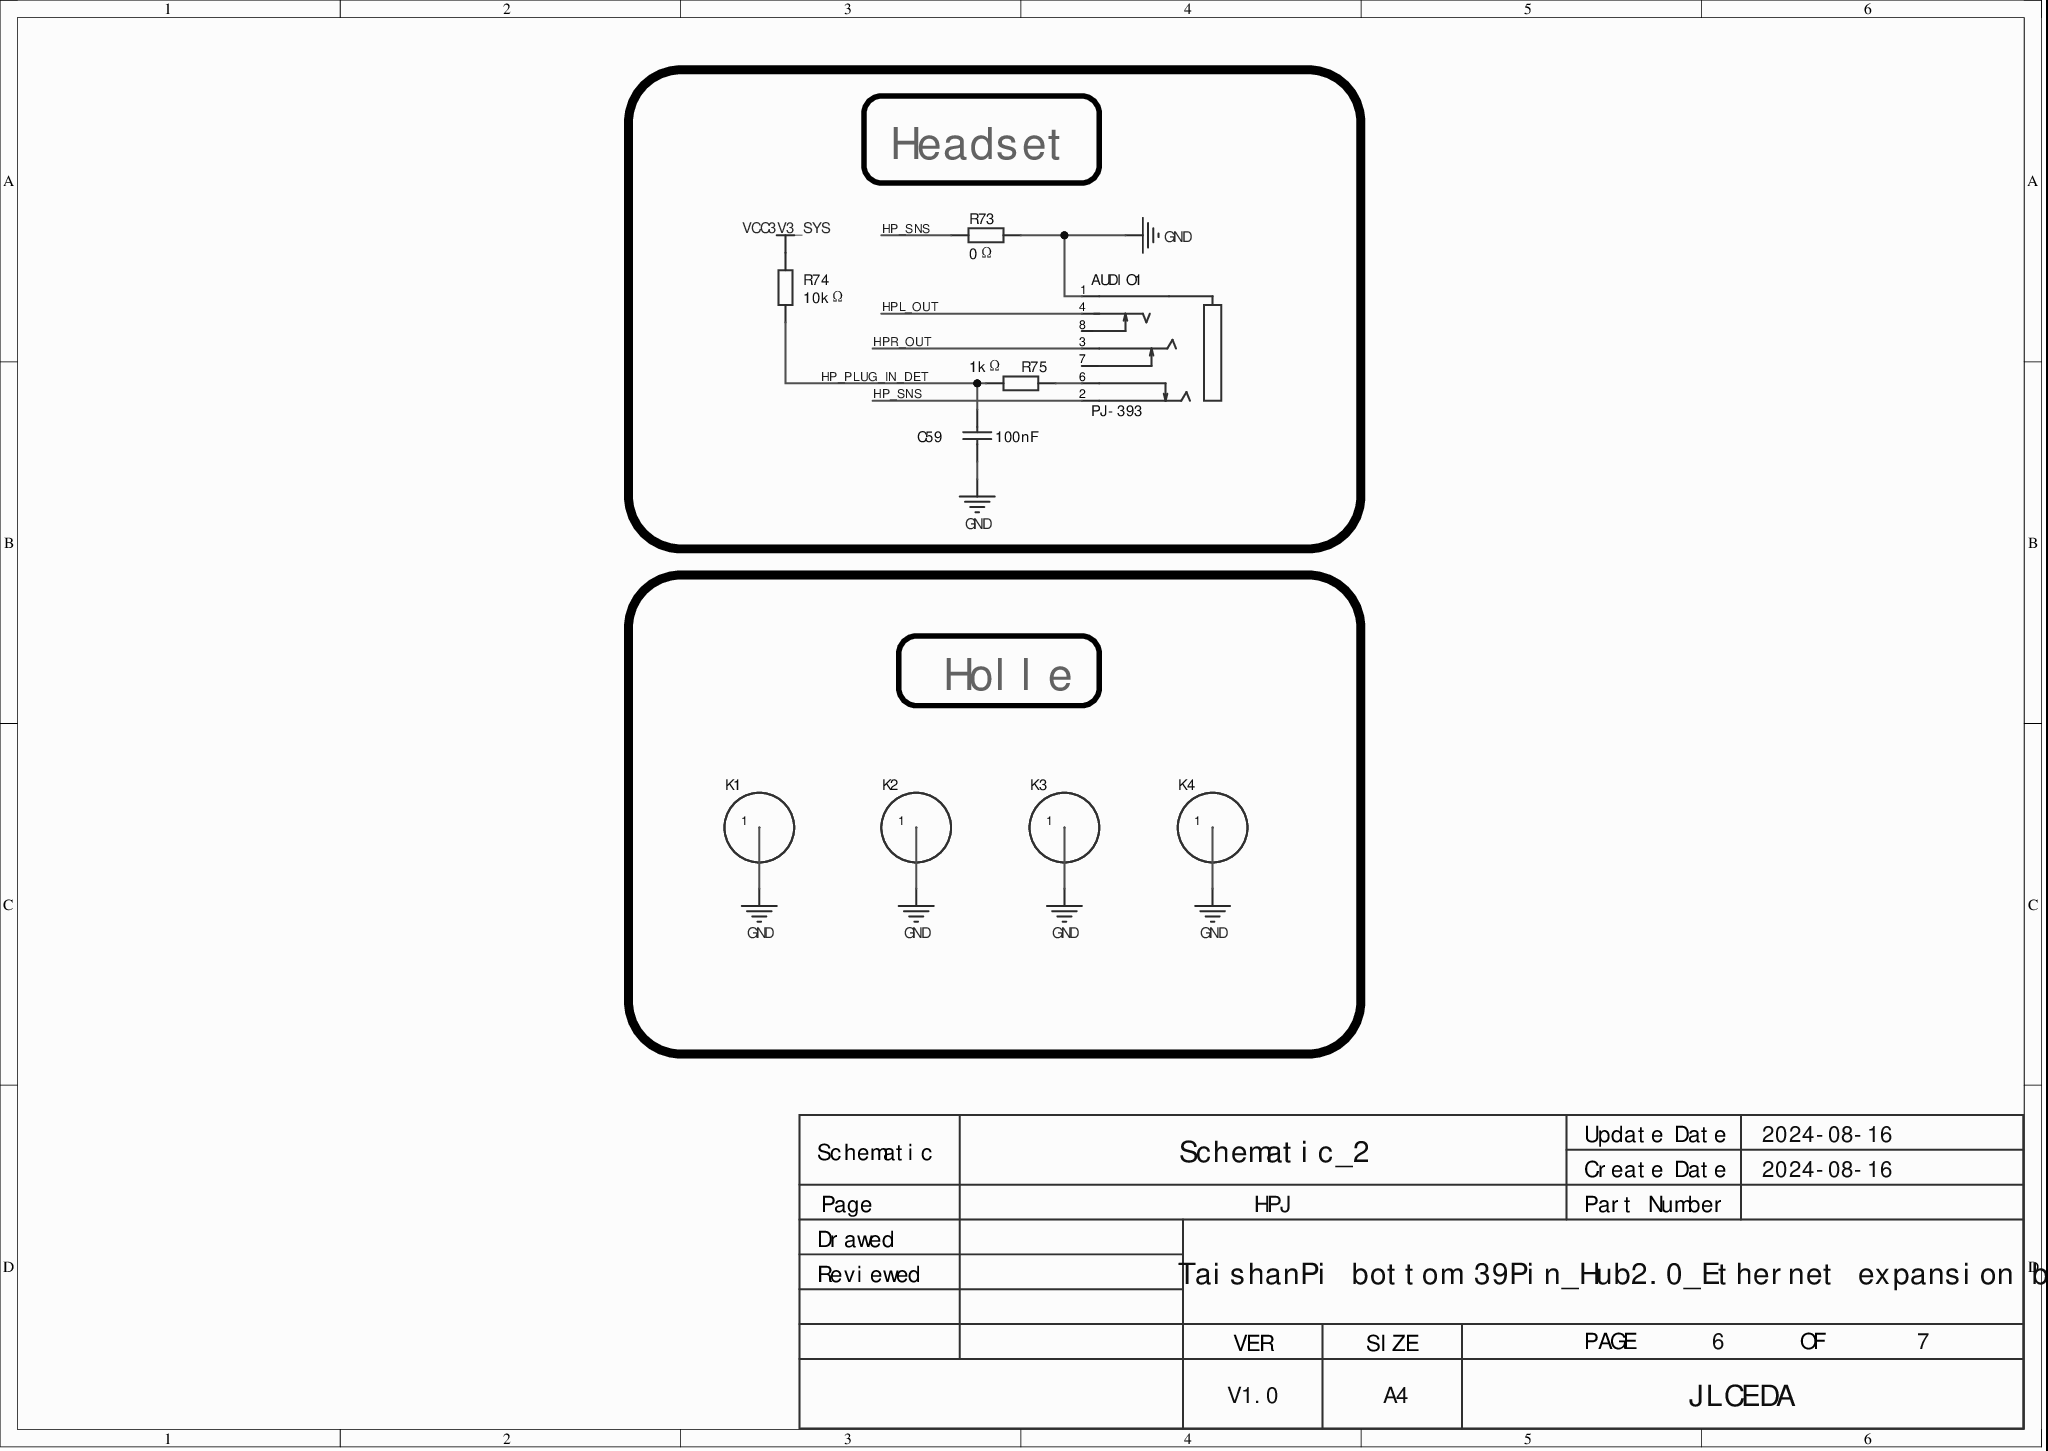
[diagram p0: MISC84334-5.SchDoc]
# Altium project MISC84334.PrjPcb (part 3 of 5)

## Sheet MISC84334-5.SchDoc
size 297 x 210 mm; Symbol: Sheet-Symbol_A4; Company: JLCEDA; Version: V1.0; Page Size: A4; @Project Name: COMPANY_A TaishanPi bottom 39Pin_Hub2.0_Ethernet expansion board; @Page Count: 7; @Update Date: 2024-08-16; @Create Date: 2024-08-16; @Schematic Name: Schematic_2; @Page No: 6; @Page Name: HPJ; Device: Sheet-Symbol_A4

### Parts
AUDIO1  PJ-393  [AUDIO-SMD_PJ-393]
C59  100nF  [R0402]
K1  (no value)  [125 X 300]
K2  (no value)  [125 X 300]
K3  (no value)  [125 X 300]
K4  (no value)  [125 X 300]
R73  0Ω  [R0402]
R74  10kΩ  [R0402]
R75  1kΩ  [R0402]

### Blocks framed on the sheet
Headset: AUDIO1 C59 R73-R75
Holle: K1-K4

### Nets
GND: AUDIO1.1 C59.2 K1.1 K2.1 K3.1 K4.1 R73.2
VCC3V3_SYS: R74.2
HP_PLUG_IN_DET: C59.1 R74.1 R75.1  [project net GPIO0_C5]
HP_SNS: AUDIO1.2 R73.1
HPL_OUT: AUDIO1.4
HPR_OUT: AUDIO1.3
NetAUDIO1_6: AUDIO1.6 R75.2

Not connected (* = marked no-connect by the designer): AUDIO1 7* 8*

### Notes on the sheet
- Update Date
- 2024-08-16
- Schematic
- Page
- Schematic_2
- HPJ
- Create Date
- Part Number
- Reviewed
- Drawed
- COMPANY_A TaishanPi bottom 39Pin_Hub2.0_Ethernet expansion board
- VER
- V1.0
- SIZE
- A4
- PAGE
- 6
- JLCEDA
- OF
- 7

### Library data of the parts
AUDIO1 = PJ-393_C2837065: Manufacturer: G-Switch(品赞); AddInBom: yes; ModelId: a1f08b2a92b045ef98fdf9ef00732f66; ModelTransform: 570.865,311.023,0,90,0,0,0.003,-29.524,-19.685; Device: PJ-393_C2837065; Symbol: PJ-393_C2837065; LCSC Part Name: 3.5mm耳机插座; SupplierPart: C2837065; ManufacturerPart: PJ-393; Supplier Footprint: SMD; JLCPCB Part Class: Extended library; Datasheet: https://atta.szlcsc.com/upload/public/pdf/source/20211203/D20F4B2397BACF41B9E43FB76A73FA52.pdf; Supplier: LCSC; ConvertToPcb: yes; FootprintName: AUDIO-SMD_PJ-393; ModelName: AUDIO-SMD_PJ-393
C59 = CL05B104KO5NNNC: Capacitance:100nF;Tolerance:±10%;Rated voltage:16V;Dielectric(Temp. coefficient):X7R;; Manufacturer: SAMSUNG(三星); AddInBom: yes; ModelId: 36a51122f27c49738f86b3bfa98863e0; ModelName: C0402_L1.0-W0.5-H0.5; ModelTransform: 39.37,19.685,0,0,0,0,0,0,0; Tolerance: ±10%; Voltage Rated: 16V; Temperature Coefficient: X7R; Device: CL05B104KO5NNNC; Symbol: CL05B104KO5NNNC; LCSC Part Name: 100nF ±10% 16V; SupplierPart: C1525; ManufacturerPart: CL05B104KO5NNNC; Supplier Footprint: 0402; JLCPCB Part Class: Basic library; Datasheet: https://atta.szlcsc.com/upload/public/pdf/source/20160103/1457707674891.pdf; Supplier: LCSC; ConvertToPcb: yes; FootprintName: R0402; Value: 100nF
K1-K4 = 125 X 300: AddInBom: yes; SymbolName: H?; Device: 125 X 300; ConvertToPcb: yes; FootprintName: 125 X 300
R73 = 0402WGF0000TCE: Resistor type:Thick film resistor;Resistance:0Ω;Tolerance:±1%;Power:62.5mW;; Manufacturer: UNI-ROYAL(厚声); AddInBom: yes; ModelId: 671aefced39d4c318694bba8bd8efd39; ModelName: R0402_L1.0-W0.5-H0.5; ModelTransform: 39.37,19.685,0,0,0,0,0,0.0005,0; Tolerance: ±1%; Power(Watts): 62.5mW; Temperature Coefficient: ±800ppm/℃; Overload Voltage (Max): 50V; Symbol: 0402WGF0000TCE; Device: 0402WGF0000TCE; Supplier: LCSC; Manufacturer Part: 0402WGF0000TCE; Supplier Part: C17168; Value: 0Ω; JLCPCB Part Class: Basic library; LCSC Part Name: 0Ω ±1% 62.5mW; Supplier Footprint: 0402; Datasheet: https://atta.szlcsc.com/upload/public/pdf/source/20200306/C422600_1E6D84923E4A46A82E41ADD87F860B5C.pdf; ConvertToPcb: yes; FootprintName: R0402; Type: Thick film resistor; Operating Temperature Range: -55℃~+155℃
R74 = 0402WGF1002TCE: Resistor type:Thick film resistor;Resistance:10kΩ;Tolerance:±1%;Power:62.5mW;Max working voltage:50V;Temp. coefficient:±100ppm/℃;; Manufacturer: UNI-ROYAL(厚声); Symbol: 0402WGF1003TCE; AddInBom: yes; ModelId: 671aefced39d4c318694bba8bd8efd39; ModelName: R0402_L1.0-W0.5-H0.5; ModelTransform: 39.37,19.685,0,0,0,0,0,0.0005,0; Tolerance: ±1%; Power(Watts): 62.5mW; Overload Voltage (Max): 50V; LCSC Part Name: 10kΩ ±1% 62.5mW 厚膜电阻; JLCPCB Part Class: Basic Part; Device: 0402WGF1002TCE; SupplierPart: C25744; ManufacturerPart: 0402WGF1002TCE; Supplier Footprint: 0402; Datasheet: https://atta.szlcsc.com/upload/public/pdf/source/20200306/C422600_1E6D84923E4A46A82E41ADD87F860B5C.pdf; Supplier: LCSC; ConvertToPcb: yes; FootprintName: R0402; Type: Thick film resistor; Value: 10kΩ; Temperature Coefficient: ±100ppm/℃; Operating Temperature Range: -55℃~+155℃
R75 = 0402WGF1001TCE: Resistor type:Thick film resistor;Resistance:1kΩ;Tolerance:±1%;Power:62.5mW;Temp. coefficient:±100ppm/℃;Max working voltage:50V;Operating temperature:-55℃~+155℃;; Manufacturer: UNI-ROYAL(厚声); AddInBom: yes; ModelId: 671aefced39d4c318694bba8bd8efd39; ModelName: R0402_L1.0-W0.5-H0.5; ModelTransform: 39.37,19.685,0,0,0,0,0,0.0005,0; Tolerance: ±1%; Power(Watts): 62.5mW; Overload Voltage (Max): 50V; Device: 0402WGF1001TCE; Symbol: 0402WGF1001TCE; LCSC Part Name: 1kΩ ±1% 62.5mW; SupplierPart: C11702; ManufacturerPart: 0402WGF1001TCE; Supplier Footprint: 0402; JLCPCB Part Class: Basic Part; Datasheet: https://atta.szlcsc.com/upload/public/pdf/source/20200306/C422600_1E6D84923E4A46A82E41ADD87F860B5C.pdf; Supplier: LCSC; ConvertToPcb: yes; FootprintName: R0402; Type: Thick film resistor; Value: 1kΩ; Temperature Coefficient: ±100ppm/℃; Operating Temperature Range: -55℃~+155℃

## Sheet MISC84334-6.SchDoc
size 297 x 210 mm; Symbol: Sheet-Symbol_A4; Company: JLCEDA; Version: V1.0; Page Size: A4; @Project Name: COMPANY_A TaishanPi bottom 39Pin_Hub2.0_Ethernet expansion board; @Page Count: 7; @Update Date: 2024-08-16; @Create Date: 2024-08-16; @Schematic Name: Schematic_2; @Page No: 5; @Page Name: PCIE; Device: Sheet-Symbol_A4
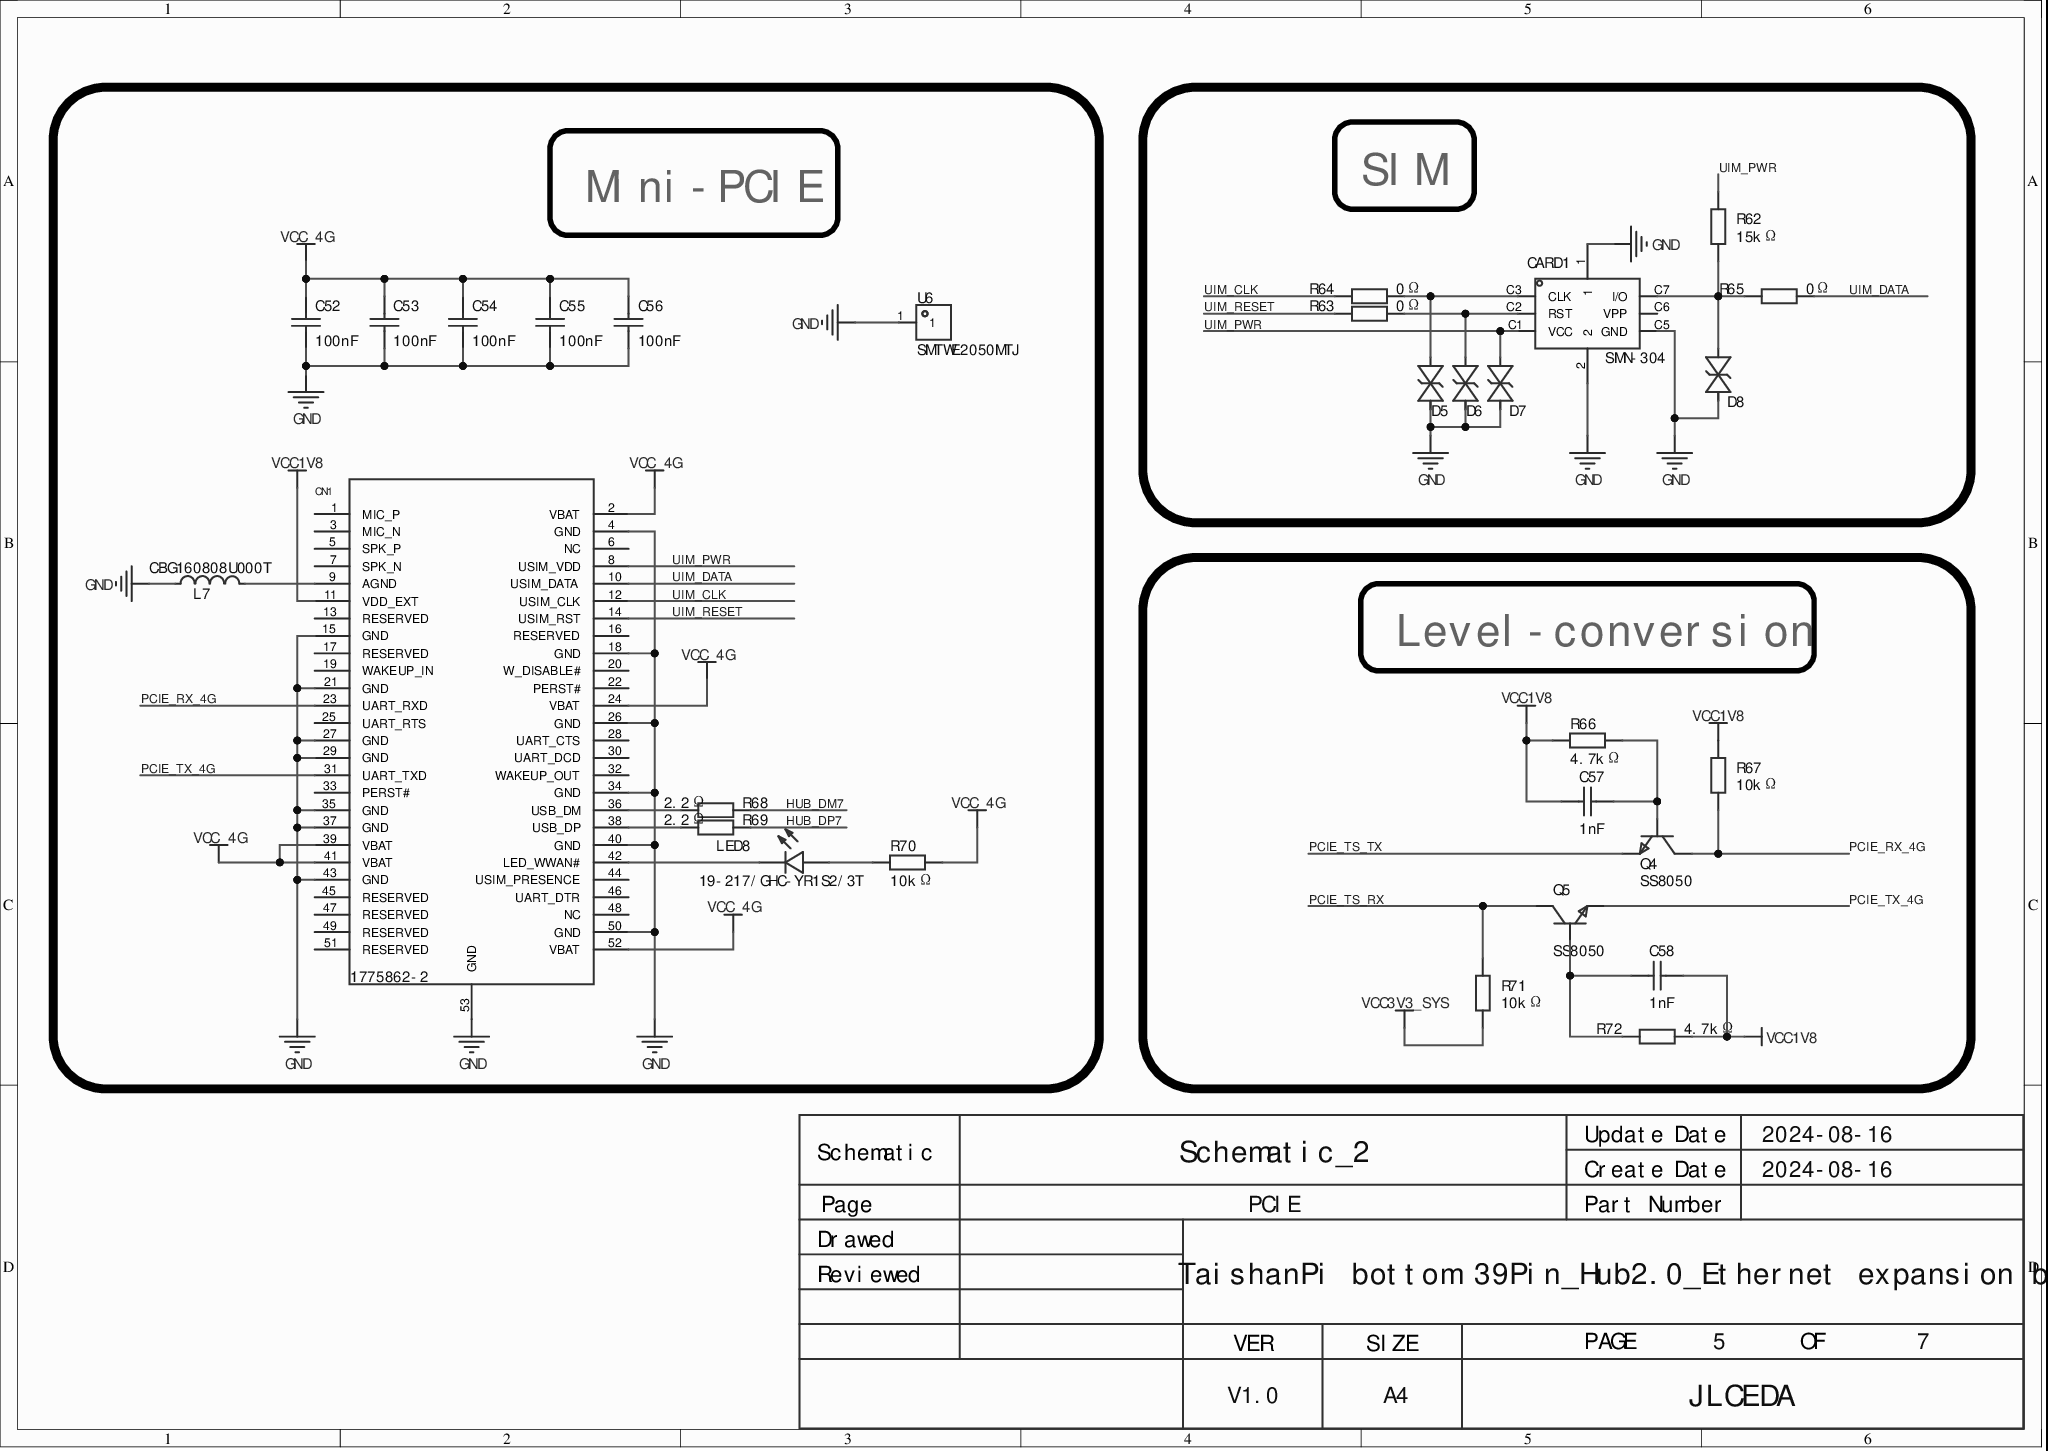
[diagram p1: MISC84334-6.SchDoc]

### Parts
C52  100nF  [R0402]
C53  100nF  [R0402]
C54  100nF  [R0402]
C55  100nF  [R0402]
C56  100nF  [R0402]
C57  1nF  [R0402]
C58  1nF  [R0402]
CARD1  SMN-304  [SIM-SMD_SMN-304]
CN1  1775862-2  [PCI-SMD_1775862-2]
D5  KLXES15AAA1  [R0402]  (value not drawn)
D6  KLXES15AAA1  [R0402]  (value not drawn)
D7  KLXES15AAA1  [R0402]  (value not drawn)
D8  KLXES15AAA1  [R0402]  (value not drawn)
L7  CBG160808U000T  [L0603]
LED8  19-217/GHC-YR1S2/3T  [LED0603-RD]
Q4  SS8050  [SOT-23-3_L2.9-W1.3-P1.90-LS2.4-BR]
Q5  SS8050  [SOT-23-3_L2.9-W1.3-P1.90-LS2.4-BR]
R62  15kΩ  [R0402]
R63  0Ω  [R0402]
R64  0Ω  [R0402]
R65  0Ω  [R0402]
R66  4.7kΩ  [R0402]
R67  10kΩ  [R0402]
R68  2.2Ω  [R0402]
R69  2.2Ω  [R0402]
R70  10kΩ  [R0402]
R71  10kΩ  [R0402]
R72  4.7kΩ  [R0402]
U6  SMTWE2050MTJ  [SMD_BD4.4-L4.4-D2.8]

### Blocks framed on the sheet
Mini-PCIE: C52-C56 CN1 L7 LED8 R68-R70 U6
SIM: CARD1 D5-D8 R62-R65
Level-conversion: C57 C58 Q4 Q5 R66 R67 R71 R72

### Nets
GND: C52.1 C53.1 C54.1 C55.1 C56.1 CARD1.1 CARD1.2 CARD1.C5(GND) CN1.4(GND) CN1.15(GND) CN1.18(GND) CN1.21(GND) CN1.26(GND) CN1.27(GND) CN1.29(GND) CN1.34(GND) CN1.35(GND) CN1.37(GND) CN1.40(GND) CN1.43(GND) CN1.50(GND) CN1.53(GND) D5.2(A) D6.2(A) D7.2(A) D8.2(A) L7.1 U6.1
VCC1V8: C57.1 C58.2 CN1.11(VDD_EXT) R66.1 R67.2 R72.2
VCC3V3_SYS: R71.1
VCC_4G: C52.2 C53.2 C54.2 C55.2 C56.2 CN1.2(VBAT) CN1.24(VBAT) CN1.39(VBAT) CN1.41(VBAT) CN1.52(VBAT) R70.2
HUB_DM7: R68.2
HUB_DP7: R69.2
PCIE_RX_4G: CN1.23(UART_RXD) Q4.3(C) R67.1
PCIE_TS_RX: Q5.3(C) R71.2
PCIE_TS_TX: Q4.2(E)
PCIE_TX_4G: CN1.31(UART_TXD) Q5.2(E)
UIM_CLK: CN1.12(USIM_CLK) R64.1
UIM_DATA: CN1.10(USIM_DATA) R65.2
UIM_PWR: CARD1.C1(VCC) CN1.8(USIM_VDD) D7.1(K) R62.2
UIM_RESET: CN1.14(USIM_RST) R63.1
NetC57_2: C57.2 Q4.1(B) R66.2
NetC58_1: C58.1 Q5.1(B) R72.1
NetCARD1_C2: CARD1.C2(RST) D6.1(K) R63.2
NetCARD1_C3: CARD1.C3(CLK) D5.1(K) R64.2
NetCARD1_C7: CARD1.C7(I/O) D8.1(K) R62.1 R65.1
NetCN1_9: CN1.9(AGND) L7.2
NetCN1_36: CN1.36(USB_DM) R68.1
NetCN1_38: CN1.38(USB_DP) R69.1
NetCN1_42: CN1.42(LED_WWAN#) LED8.1(C)
NetLED8_2: LED8.2(A) R70.1

Not connected (* = marked no-connect by the designer): CARD1 C6(VPP)*; CN1 1(MIC_P)* 3(MIC_N)* 5(SPK_P)* 6(NC)* 7(SPK_N)* 13(RESERVED)* 16(RESERVED)* 17(RESERVED)* 19(WAKEUP_IN)* 20(W_DISABLE#)* 22(PERST#)* 25(UART_RTS)* 28(UART_CTS)* 30(UART_DCD)* 32(WAKEUP_OUT)* 33(PERST#)* 44(USIM_PRESENCE)* 45(RESERVED)* 46(UART_DTR)* 47(RESERVED)* 48(NC)* 49(RESERVED)* 51(RESERVED)*

### Notes on the sheet
- Update Date
- 2024-08-16
- Schematic
- Page
- Schematic_2
- PCIE
- Create Date
- Part Number
- Reviewed
- Drawed
- COMPANY_A TaishanPi bottom 39Pin_Hub2.0_Ethernet expansion board
- VER
- V1.0
- SIZE
- A4
- PAGE
- 5
- JLCEDA
- OF
- 7

### Library data of the parts
C52-C56 = CL05B104KO5NNNC: as C59 on sheet MISC84334-5; Device: CL05B104KO5NNNC; Symbol: CL05B104KO5NNNC; LCSC Part Name: 100nF ±10% 16V; SupplierPart: C1525; ManufacturerPart: CL05B104KO5NNNC; Supplier Footprint: 0402; JLCPCB Part Class: Basic library; Datasheet: https://atta.szlcsc.com/upload/public/pdf/source/20160103/1457707674891.pdf; Supplier: LCSC; ConvertToPcb: yes; FootprintName: R0402; Value: 100nF
C57 C58 = CC0402KRX7R9BB102: Capacitance:1nF;Tolerance:±10%;Rated voltage:50V;Dielectric(Temp. coefficient):X7R;; Manufacturer: YAGEO(国巨); AddInBom: yes; ModelId: 36a51122f27c49738f86b3bfa98863e0; ModelName: C0402_L1.0-W0.5-H0.5; ModelTransform: 39.37,19.685,0,0,0,0,0,0,0; Tolerance: ±10%; Voltage Rated: 50V; Temperature Coefficient: X7R; Symbol: CC0402KRX7R9BB102; Device: CC0402KRX7R9BB102; Supplier: LCSC; Manufacturer Part: CC0402KRX7R9BB102; Value: 1nF; Supplier Part: C106205; JLCPCB Part Class: Extended library; LCSC Part Name: 1nF ±10% 50V; Supplier Footprint: 0402; Datasheet: https://atta.szlcsc.com/upload/public/pdf/source/20171226/C106205_15142609593391205665.pdf; ConvertToPcb: yes; FootprintName: R0402
CARD1 = SMN-304: Card insertion:Push-pull;Card type:NanoSIM card;Connector type:Card holder;Max body height:1.35mm;Contact material:-;Contact plating:Gold;Operating temperature:-40℃~+85℃;Soldering temperature (max):260℃;; Manufacturer: XUNPU(讯普); AddInBom: yes; ModelId: 4b378b9bec8c4fef9fa08472d3a8fc13; ModelTransform: 447.6369,484.251,0,0,0,0,0,0,0; Body Height (Max): 1.35mm; Welding Temperature (Max): 260℃; Device: SMN-304; Symbol: SMN-304; LCSC Part Name: 拔插式 NanoSIM卡 卡座; SupplierPart: C266889; ManufacturerPart: SMN-304; Supplier Footprint: SMD; JLCPCB Part Class: Extended library; Datasheet: https://atta.szlcsc.com/upload/public/pdf/source/20210906/008C96EE0BDD3DBC40121ECB56D55849.pdf; Supplier: LCSC; ConvertToPcb: yes; FootprintName: SIM-SMD_SMN-304; ModelName: SIM-SMD_SMN-304; Card Connection Mode: Push-pull; Card Type: NanoSIM card; Connector Type: Card holder; Contact Material: -; Contact Plating: Gold; Operating Temperature Range: -40℃~+85℃
CN1 = 1775862-2: Connector type:mSATA; mPCI-E;Pitch:0.8mm;Total pins:52;Mounting:Horizontal SMD;Operating temperature:-;; Manufacturer: TE Connectivity(美国泰科); NO_CONNECT: yes; ModelId: ab3b7804cc444411a8fc86f49fede5b5; ModelTransform: 1177.163,357.4796,0,0,0,0,0,3.937,-23.622; Symbol: 1775862-2; Device: 1775862-2; Supplier: LCSC; SupplierPart: C428486; ManufacturerPart: 1775862-2; JLCPCB Part Class: Extended Part; FootprintName: PCI-SMD_1775862-2; ModelName: PCI-SMD_1775862-2
D5-D8 = KLXES15AAA1: Polarity:Bidirectional;Reverse standoff voltage(Vrwm):5V;Clamping voltage(Vc)@Ipp:40V;; Manufacturer: KUU; AddInBom: yes; ModelId: 62a80a189f1b46df8ba79817b730b378; ModelName: D0402_L1.0-W0.5-H0.5; ModelTransform: 39.37,19.685,0,0,0,0,0,0,0; Reverse Stand-Off Voltage (Vrwm): 5V; Clamping Voltage@Ipp: 40V; Device: KLXES15AAA1; Symbol: KLXES15AAA1; LCSC Part Name: KLXES15AAA1; SupplierPart: C2892490; ManufacturerPart: KLXES15AAA1; Supplier Footprint: 0402; JLCPCB Part Class: Extended Part; Datasheet: https://atta.szlcsc.com/upload/public/pdf/source/20210908/40FD94D5521B4EF0ED53BC030E77ED53.pdf; Supplier: LCSC; ConvertToPcb: yes; FootprintName: R0402; Polarity: Bidirectional
L7 = CBG160808U000T: Impedance@test frequency:0Ω@100MHz;DC resistance(RDC):100mΩ;; Manufacturer: FH(风华); AddInBom: yes; ModelId: 2bc5ec593d464d6ba9807aec0b5673c2; ModelName: L0603_L1.6-W0.8-H0.5_BEAD; ModelTransform: 62.992,31.496,0,180,0,0,0.094,0.629,0; DC Resistance: 100mΩ; Current Rating: 800mA; Circuits: 1; Device: CBG160808U000T; Symbol: CBG160808U000T; LCSC Part Name: 单路 0603磁珠 阻抗0Ω@100MHz; SupplierPart: C43163; ManufacturerPart: CBG160808U000T; Supplier Footprint: 0603; Datasheet: https://atta.szlcsc.com/upload/public/pdf/source/20151026/1457707503572.pdf; Supplier: LCSC; ConvertToPcb: yes; FootprintName: L0603; Impedance @ Frequency: 0Ω@100MHz
LED8 = 19-217/GHC-YR1S2/3T: Emitting color:Emerald green;Diode configuration:-;Dominant wavelength:520nm~535nm;Color temp.:-;Power:110mW;Mounting:-;; Manufacturer: EVERLIGHT(亿光); AddInBom: yes; ModelId: 1f0d29a91be547639d425604e9b96ebb; ModelTransform: 63.7794,32.283,0,0,0,0,0,0,0; Lens Color: Water clear; Peak Wavelength: 518nm; Forward Current: 20mA; Power Dissipation: 110mW; Viewing Angle: 120°; Device: 19-217/GHC-YR1S2/3T; Symbol: 19-217/GHC-YR1S2/3T; LCSC Part Name: 19-217/GHC-YR1S2/3T; SupplierPart: C72043; ManufacturerPart: 19-217/GHC-YR1S2/3T; Supplier Footprint: 0603; JLCPCB Part Class: Basic Part; Datasheet: https://atta.szlcsc.com/upload/public/pdf/source/20160507/1462613613780.pdf; Supplier: LCSC; ConvertToPcb: yes; FootprintName: LED0603-RD; ModelName: LED0603-RD; Emitted Color: Emerald green; Diode Configuration: -; Dominant Wavelength: 520nm~535nm; Color Temperature: -; Mounting Sytle: -; Operating Temperature: -40℃~+85℃
Q4 Q5 = SS8050_C2150: Transistor type:NPN;collector current(Ic):1.5A;Vce breakdown voltage(Vceo):25V;Power(Pd):300mW;DC current gain(hFE@Ic,Vce):200@100mA,1V;; Manufacturer: CJ(江苏长电/长晶); AddInBom: yes; ModelId: c62791f0466c4ae2a892c056b845b0ca; ModelName: SOT-23-3P_L2.9-W1.3-H1.0-LS2.4-P0.95; ModelTransform: 98.425,114.173,0,180,0,0,0.0005,-0.0005,0; Transistor Type: NPN; Collector Current (Ic): 1.5A; Collector-Emitter Breakdown Voltage (Vceo): 25V; Power Dissipation (Pd): 300mW; Transition Frequency (fT): 100MHz; Collector Cut-Off Current (Icbo): 100nA; Collector-Emitter Saturation Voltage (VCE(sat)@Ic,Ib): 500mV@800mA,80mA; Symbol: SS8050_C2150; Device: SS8050_C2150; Supplier: LCSC; Manufacturer Part: SS8050; Supplier Part: C2150; LCSC Part Name: 耐压:25V 电流:1.5A NPN hfe=200~350; Supplier Footprint: SOT-23; Datasheet: https://atta.szlcsc.com/upload/public/pdf/source/20230322/AEE86F4B043774EFF80CAEA14A37D9E9.pdf; ConvertToPcb: yes; FootprintName: SOT-23-3_L2.9-W1.3-P1.90-LS2.4-BR; DC Current Gain (hFE@Ic,Vce): 200@100mA,1V; Operating Temperature: +150℃@(Tj)
R62 = 0402WGF1502TCE: Resistor type:Thick film resistor;Resistance:15kΩ;Tolerance:±1%;Power:62.5mW;; Manufacturer: UNI-ROYAL(厚声); AddInBom: yes; ModelId: 671aefced39d4c318694bba8bd8efd39; ModelName: R0402_L1.0-W0.5-H0.5; ModelTransform: 39.37,19.685,0,0,0,0,0,0.0005,0; Tolerance: ±1%; Power(Watts): 62.5mW; Temperature Coefficient: ±100ppm/℃; Overload Voltage (Max): 50V; Device: 0402WGF1502TCE; Symbol: 0402WGF1502TCE; LCSC Part Name: 15kΩ ±1% 62.5mW; SupplierPart: C25756; ManufacturerPart: 0402WGF1502TCE; Supplier Footprint: 0402; JLCPCB Part Class: Basic library; Datasheet: https://atta.szlcsc.com/upload/public/pdf/source/20200306/C422600_1E6D84923E4A46A82E41ADD87F860B5C.pdf; Supplier: LCSC; ConvertToPcb: yes; FootprintName: R0402; Type: Thick film resistor; Value: 15kΩ; Operating Temperature Range: -55℃~+155℃
R63-R65 = 0402WGF0000TCE: as R73 on sheet MISC84334-5; Symbol: 0402WGF0000TCE; Device: 0402WGF0000TCE; Supplier: LCSC; Manufacturer Part: 0402WGF0000TCE; Supplier Part: C17168; Value: 0Ω; JLCPCB Part Class: Basic library; LCSC Part Name: 0Ω ±1% 62.5mW; Supplier Footprint: 0402; Datasheet: https://atta.szlcsc.com/upload/public/pdf/source/20200306/C422600_1E6D84923E4A46A82E41ADD87F860B5C.pdf; ConvertToPcb: yes; FootprintName: R0402; Type: Thick film resistor; Operating Temperature Range: -55℃~+155℃
R66 R72 = 0402WGF4701TCE: Resistor type:Thick film resistor;Resistance:4.7kΩ;Tolerance:±1%;Power:62.5mW;; Manufacturer: UNI-ROYAL(厚声); AddInBom: yes; ModelId: 671aefced39d4c318694bba8bd8efd39; ModelName: R0402_L1.0-W0.5-H0.5; ModelTransform: 39.37,19.685,0,0,0,0,0,0.0005,0; Tolerance: ±1%; Power(Watts): 62.5mW; Temperature Coefficient: ±100ppm/℃; Overload Voltage (Max): 50V; Symbol: 0402WGF4701TCE; Device: 0402WGF4701TCE; Supplier: LCSC; Manufacturer Part: 0402WGF4701TCE; Supplier Part: C25900; Value: 4.7kΩ; JLCPCB Part Class: Basic library; LCSC Part Name: 4.7kΩ ±1% 62.5mW; Supplier Footprint: 0402; Datasheet: https://atta.szlcsc.com/upload/public/pdf/source/20200306/C422600_1E6D84923E4A46A82E41ADD87F860B5C.pdf; ConvertToPcb: yes; FootprintName: R0402; Type: Thick film resistor; Operating Temperature Range: -55℃~+155℃
R67 R71 = 0402WGF1002TCE: Resistor type:Thick film resistor;Resistance:10kΩ;Tolerance:±1%;Power:62.5mW;; Manufacturer: UNI-ROYAL(厚声); AddInBom: yes; ModelId: 671aefced39d4c318694bba8bd8efd39; ModelName: R0402_L1.0-W0.5-H0.5; ModelTransform: 39.37,19.685,0,0,0,0,0,0.0005,0; Tolerance: ±1%; Power(Watts): 62.5mW; Temperature Coefficient: ±100ppm/℃; Overload Voltage (Max): 50V; Symbol: 0402WGF1002TCE; Device: 0402WGF1002TCE; Supplier: LCSC; Manufacturer Part: 0402WGF1002TCE; Supplier Part: C25744; Value: 10kΩ; JLCPCB Part Class: Basic library; LCSC Part Name: 10kΩ ±1% 62.5mW; Supplier Footprint: 0402; Datasheet: https://atta.szlcsc.com/upload/public/pdf/source/20200306/C422600_1E6D84923E4A46A82E41ADD87F860B5C.pdf; ConvertToPcb: yes; FootprintName: R0402; Type: Thick film resistor; Operating Temperature Range: -55℃~+155℃
R68 R69 = 0402WGJ022JTCE: Resistor type:Thick film resistor;Resistance:2.2Ω;Tolerance:±5%;Power:62.5mW;; Manufacturer: UNI-ROYAL(厚声); AddInBom: yes; ModelId: 671aefced39d4c318694bba8bd8efd39; ModelName: R0402_L1.0-W0.5-H0.5; ModelTransform: 39.37,19.685,0,0,0,0,0,0.0005,0; Tolerance: ±5%; Power(Watts): 62.5mW; Temperature Coefficient: ±200ppm/℃; Overload Voltage (Max): 50V; Device: 0402WGJ022JTCE; Symbol: 0402WGJ022JTCE; LCSC Part Name: 2.2Ω ±5% 62.5mW; SupplierPart: C25158; ManufacturerPart: 0402WGJ022JTCE; Supplier Footprint: 0402; JLCPCB Part Class: Extended library; Datasheet: https://atta.szlcsc.com/upload/public/pdf/source/20200306/C422600_1E6D84923E4A46A82E41ADD87F860B5C.pdf; Supplier: LCSC; ConvertToPcb: yes; FootprintName: R0402; Type: Thick film resistor; Value: 2.2Ω; Operating Temperature Range: -55℃~+155℃